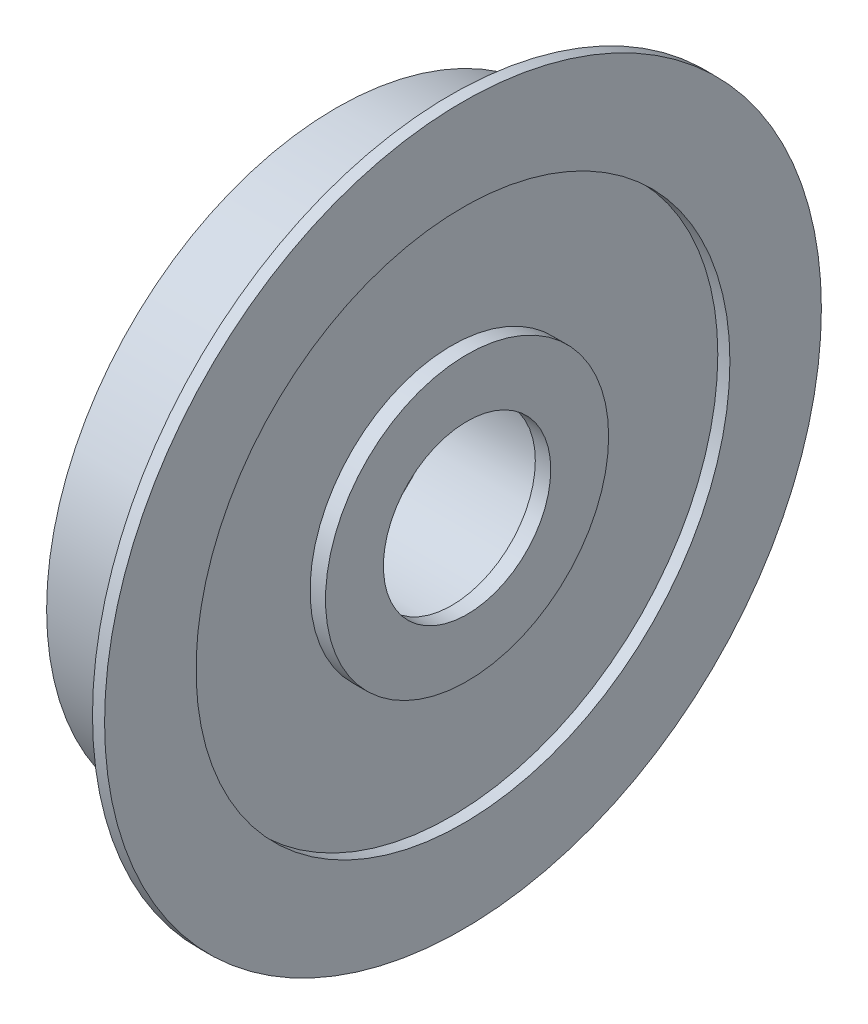
from build123d import *

# Parameters (mm, degrees)
SKETCH1_W = 1.306852865
SKETCH1_H = 4.907189237


with BuildPart() as part:
    # Sketch1 → Revolve1 (revolve)
    with BuildSketch(Plane.XY, mode=Mode.PRIVATE) as revolve1_sk:
        Polygon((108, 30.376137781), (108, 24.55), (98.286326817, 24.55), (98.286326817, 8.659632807), (108, 8.659632807), (108, 22.623174238), (109.025432246, 22.623174238), (109.025432246, 30.376137781), align=None)
        with Locations((108.718162295, 9.545177183)):
            Rectangle(SKETCH1_W, SKETCH1_H)
    revolve(revolve1_sk.sketch.rotate(Axis((0, 0, 0), (-1, 0, 0)), 90), axis=Axis((0, 0, 0), (-1, 0, 0)))


solid = part.part
